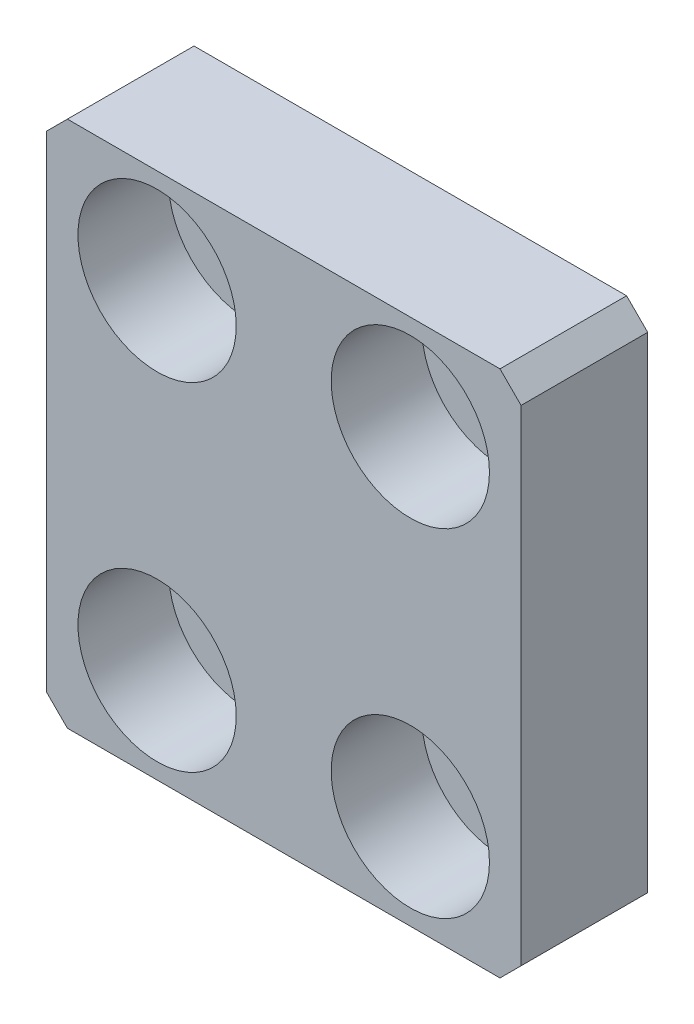
from build123d import *

# Parameters (mm, degrees)
SKETCH1_W                                           = 45
SKETCH1_H                                           = 50
BOSS_EXTRUDE1_DEPTH                                 = 12
CBORE_FOR_M8_HEX_SOCKET_HEAD_CAP_SCREW1_D           = 9
CBORE_FOR_M8_HEX_SOCKET_HEAD_CAP_SCREW1_CBORE_D     = 15
CBORE_FOR_M8_HEX_SOCKET_HEAD_CAP_SCREW1_CBORE_DEPTH = 8.6
CHAMFER1_SIZE                                       = 2


with BuildPart() as part:
    # Sketch1 → Boss-Extrude1 (new body)
    with BuildSketch(Plane.XY):
        Rectangle(SKETCH1_W, SKETCH1_H)
    extrude(amount=BOSS_EXTRUDE1_DEPTH)

    # CBORE for M8 Hex Socket Head Cap Screw1 (through all)
    with Locations(Plane.XY.offset(12)):
        with Locations((-12, 16), (12, 16), (12, -16), (-12, -16)):
            CounterBoreHole(CBORE_FOR_M8_HEX_SOCKET_HEAD_CAP_SCREW1_D / 2, CBORE_FOR_M8_HEX_SOCKET_HEAD_CAP_SCREW1_CBORE_D / 2, CBORE_FOR_M8_HEX_SOCKET_HEAD_CAP_SCREW1_CBORE_DEPTH)

    # Chamfer1
    chamfer1_edges = [part.edges().sort_by_distance(p)[0] for p in [
        (22.5, -25, 6),
        (-22.5, -25, 6),
        (-22.5, 25, 6),
        (22.5, 25, 6),
    ]]
    chamfer(chamfer1_edges, length=CHAMFER1_SIZE)


solid = part.part
